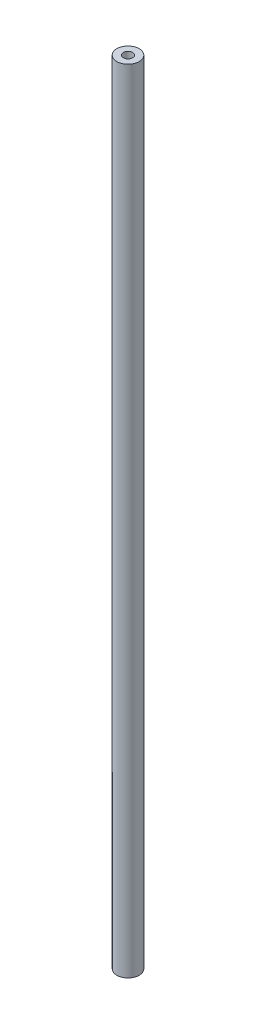
SolidWorks part; units mm, degrees
material "ABS"
ref_plane "Front Plane" through (0, 0, 0) normal (0, 0, 1) x (1, 0, 0)
ref_plane "Top Plane" through (0, 0, 0) normal (0, 1, 0) x (1, 0, 0)
ref_plane "Right Plane" through (0, 0, 0) normal (1, 0, 0) x (0, 0, -1)
sketch "Sketch1" plane through (0, 0, 0) normal (0, 0, 1) x (1, 0, 0)
  line L0 (0, -6.4416) -> (0, 89.5755) construction
  line L2 (-0.5, 0) -> (-1.2, 0)
  line L3 (-0.5, 0) -> (-0.5, 85)
  line L4 (-0.5, 85) -> (-1.2, 85)
  line L5 (-1.2, 0) -> (-1.2, 85)
  dimension "D1" = 2.4
  dimension "D2" = 85
  dimension "D3" = 1
revolve "Revolve1" add sketch "Sketch1" angle 360 about L0
